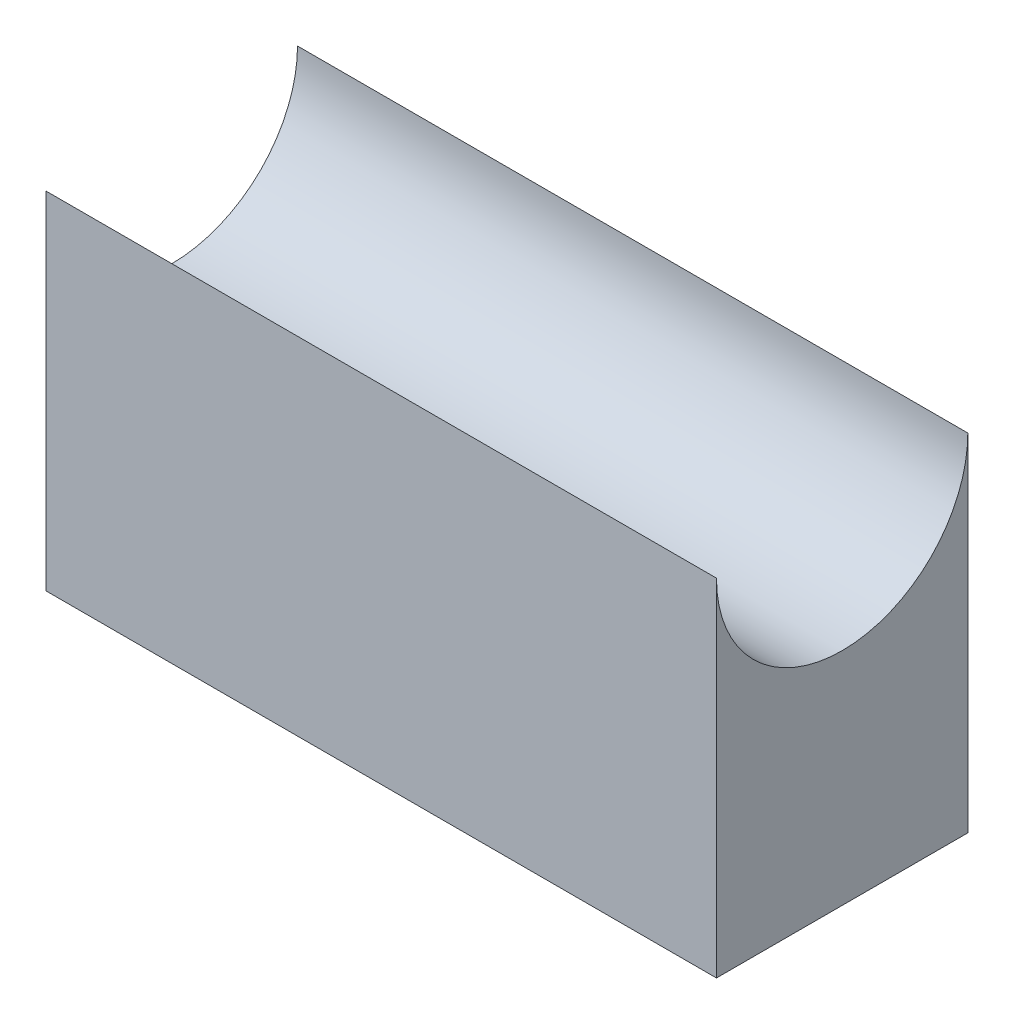
SolidWorks part; units mm, degrees
ref_plane "Front Plane" through (0, 0, 0) normal (0, 0, 1) x (1, 0, 0)
ref_plane "Top Plane" through (0, 0, 0) normal (0, 1, 0) x (1, 0, 0)
ref_plane "Right Plane" through (0, 0, 0) normal (1, 0, 0) x (0, 0, -1)
sketch "Sketch1" plane through (0, 0, 0) normal (0, 1, 0) x (1, 0, 0)
  line L1 (-40, 15) -> (40, 15)
  line L2 (-40, 15) -> (-40, -15)
  line L3 (-40, -15) -> (40, -15)
  line L4 (40, 15) -> (40, -15)
  line L5 (-40, 15) -> (40, -15) construction
  line L6 (-40, -15) -> (40, 15) construction
  point P0 (0, 0)
  dimension "D1" = 80
  dimension "D2" = 30
extrude "Boss-Extrude1" add sketch "Sketch1" along normal blind 10
sketch "Sketch3" plane through (-40, 0, 0) normal (-1, 0, 0) x (0, 0, 1)
  line L0 (-15, 10) -> (-15, 41.3303)
  line L1 (0, 28.6068) -> (0, -15.6244) construction
  line L2 (15, 10) -> (15, 41.3303)
  line L3 (-15, 10) -> (15, 10)
  arc A0 (-15, 41.3303) -> (15, 41.3303) centre (0, 41.3303) ccw
extrude "Boss-Extrude2" add sketch "Sketch3" against normal blind 80
